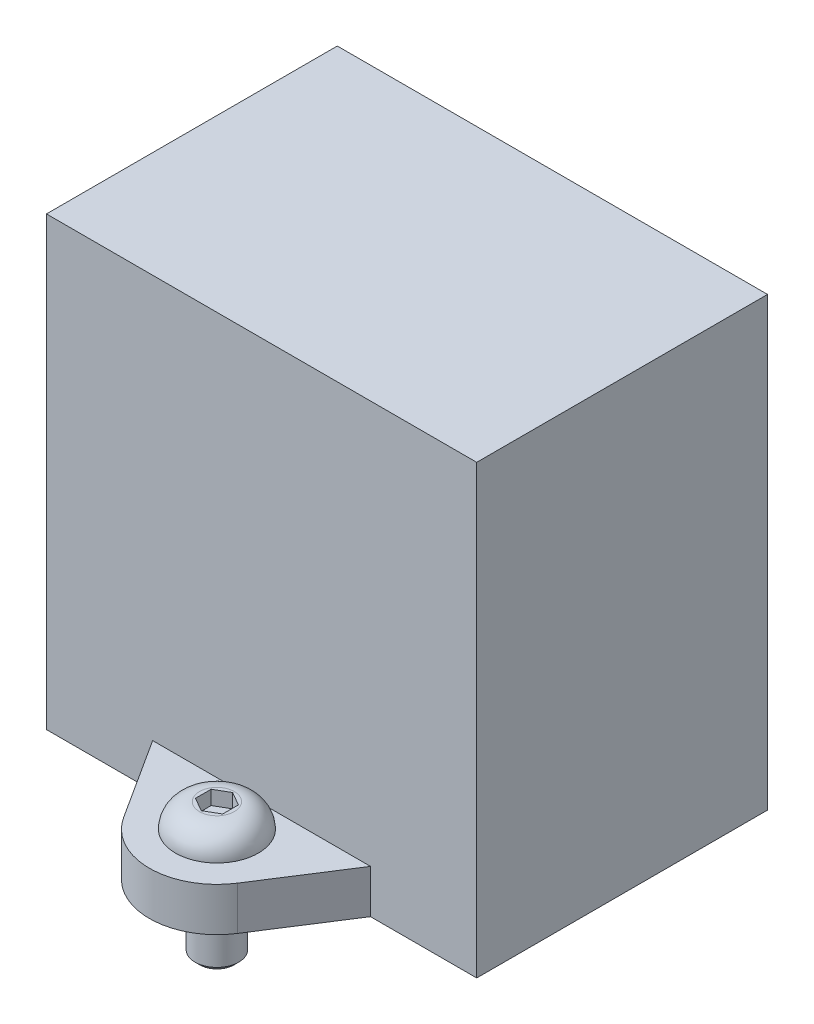
from build123d import *

# Parameters (mm, degrees)
SKETCH_1_W          = 39.5
SKETCH_1_H          = 26.7
EXTRUDE_1_DEPTH     = 41
EXTRUDE_2_DEPTH     = 4
SKETCH_3_W          = 2.15
SKETCH_3_H          = 4
CUT_EXTRUDE_1_DEPTH = 1.3


with BuildPart() as part:
    # 草图1 → 凸台-拉伸1 (new body)
    with BuildSketch(Plane(origin=(0, 0, 0), x_dir=(1, 0, 0), z_dir=(0, 1, 0))):
        with Locations((0, 13.35)):
            Rectangle(SKETCH_1_W, SKETCH_1_H)
    extrude(amount=EXTRUDE_1_DEPTH)

    # 草图2 → 凸台-拉伸2 (add)
    with BuildSketch(Plane(origin=(0, 0, 0), x_dir=(1, 0, 0), z_dir=(0, 1, 0))):
        with BuildLine():
            Line((-10, 0), (-5.217320496, -7.449562186))
            ThreePointArc((-5.217320496, -7.449562186), (0, -10.3), (5.217320496, -7.449562186))
            Line((5.217320496, -7.449562186), (10, 0))
            Line((10, 0), (-10, 0))
        make_face()
    extrude(amount=EXTRUDE_2_DEPTH)

    # 草图3 → 切除-旋转1 (revolve, cut)
    with BuildSketch(Plane.XY.offset(4.1), mode=Mode.PRIVATE) as cut_revolve_1_sk:
        with Locations((1.075, 2)):
            Rectangle(SKETCH_3_W, SKETCH_3_H)
    revolve(cut_revolve_1_sk.sketch.rotate(Axis((0, 0, 4.1), (0, 1, 0)), 270), axis=Axis((0, 0, 4.1), (0, 1, 0)), mode=Mode.SUBTRACT)

    # 草图4 → 旋转1 (revolve)
    with BuildSketch(Plane.XY.offset(4.1), mode=Mode.PRIVATE) as revolve_1_sk:
        with BuildLine():
            Line((0, 6.2), (1.6, 6.2))
            ThreePointArc((1.6, 6.2), (3.155634919, 5.555634919), (3.8, 4))
            Line((3.8, 4), (2, 4))
            Line((2, 4), (2, -5.5705))
            Line((2, -5.5705), (1.5705, -6))
            Line((1.5705, -6), (0, -6))
            Line((0, -6), (0, 6.2))
        make_face()
    revolve(revolve_1_sk.sketch.rotate(Axis((0, -6, 4.1), (0, 1, 0)), 270), axis=Axis((0, -6, 4.1), (0, 1, 0)))

    # 草图5 → 切除-拉伸1 (cut)
    with BuildSketch(Plane(origin=(0, 6.2, 0), x_dir=(1, 0, 0), z_dir=(0, 1, 0))):
        Polygon((-1.25, -3.378312164), (-1.25, -4.821687836), (0, -5.543375673), (1.25, -4.821687836), (1.25, -3.378312164), (0, -2.656624327), align=None)
    extrude(amount=-CUT_EXTRUDE_1_DEPTH, mode=Mode.SUBTRACT)


solid = part.part
